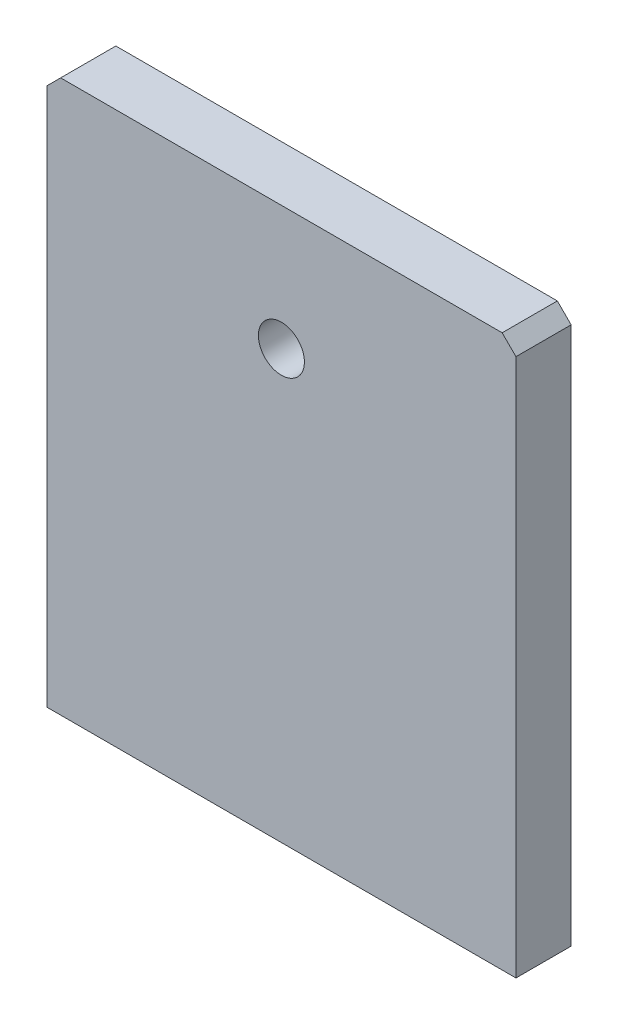
from build123d import *

# Parameters (mm, degrees)
BOSS_EXTRUDE1_DEPTH     = 20
F_3_4_10_TAPPED_HOLE1_D = 16.66748


with BuildPart() as part:
    # Sketch1 → Boss-Extrude1 (new body)
    with BuildSketch(Plane.XY):
        Polygon((0, 195), (5, 200), (165, 200), (170, 195), (170, 0), (0, 0), align=None)
    extrude(amount=BOSS_EXTRUDE1_DEPTH)

    # 3/4-10 Tapped Hole1 (through all)
    with Locations(Plane(origin=(85, 155, 20), x_dir=(1, 0, 0), z_dir=(0, 0, 1))):
        with Locations((0, 0)):
            Hole(F_3_4_10_TAPPED_HOLE1_D / 2)


solid = part.part
